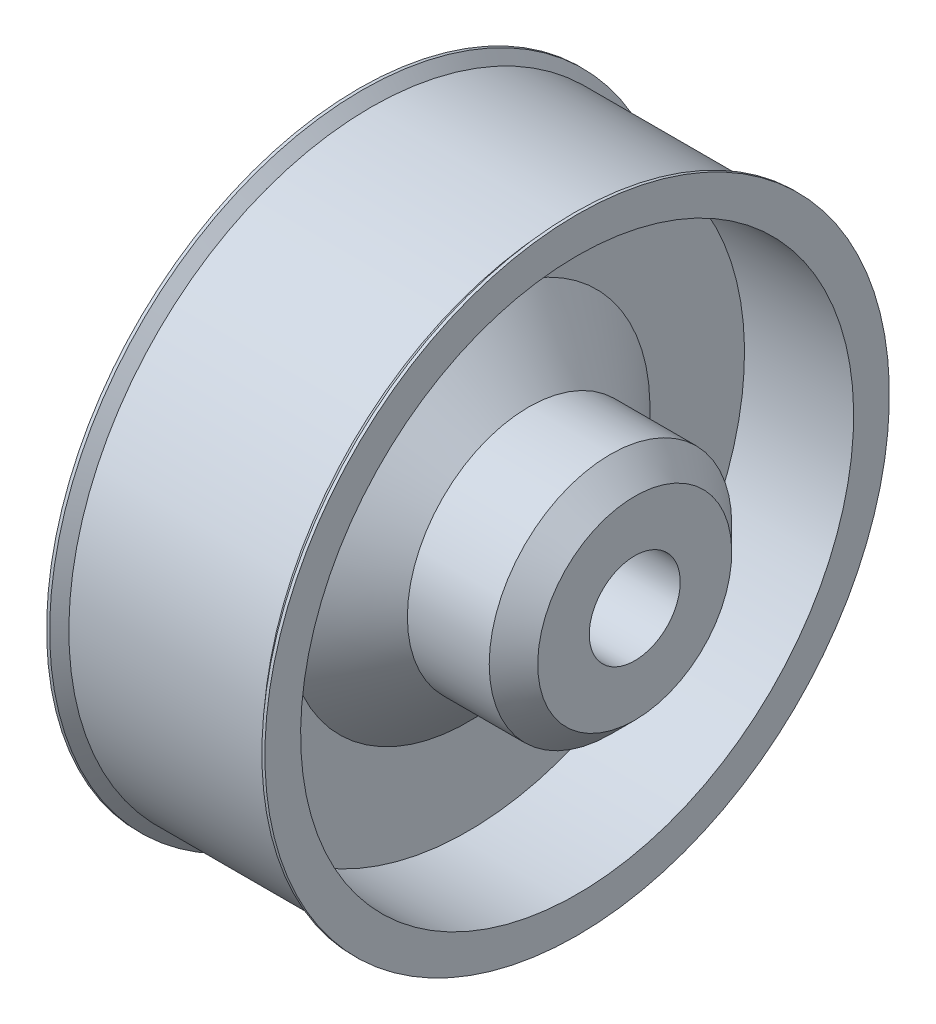
from build123d import *

# Parameters (mm, degrees)
CHAMFER1_SIZE       = 0.4
FILLET1_R           = 0.2
CHAMFER2_SIZE       = 1
BOSS_EXTRUDE1_DEPTH = 0.15
CIRPATTERN1_COUNT   = 8
BOSS_EXTRUDE2_DEPTH = 0.15
CIRPATTERN2_COUNT   = 5


with BuildPart() as part:
    # Sketch1 → Revolve1 (revolve)
    with BuildSketch(Plane.XY):
        with BuildLine():
            Line((0, 0), (0, 0.375))
            Line((0, 0.375), (1.05, 0.6))
            Line((1.05, 0.6), (1.05, 1.29376941))
            ThreePointArc((1.05, 1.29376941), (0.990535118, 1.473053702), (0.835714286, 1.581263864))
            ThreePointArc((0.835714286, 1.581263864), (0.3, 2.3), (0.835714286, 3.018736136))
            ThreePointArc((0.835714286, 3.018736136), (0.990535118, 3.126946298), (1.05, 3.30623059))
            Line((1.05, 3.30623059), (1.05, 4.231193843))
            ThreePointArc((1.05, 4.231193843), (0.953516085, 4.46412662), (0.720583307, 4.560610535))
            Line((0.720583307, 4.560610535), (0, 4.560610535))
            Line((0, 4.560610535), (0, 5.15))
            Line((0, 5.15), (0.05, 5.15))
            Line((0.05, 5.15), (0.2, 4.982919745))
            Line((0.2, 4.982919745), (3.4, 4.982919745))
            Line((3.4, 4.982919745), (3.55, 5.15))
            Line((3.55, 5.15), (3.6, 5.15))
            Line((3.6, 5.15), (3.6, 4.560610535))
            Line((3.6, 4.560610535), (1.8, 4.560610535))
            Line((1.8, 4.560610535), (1.8, 2))
            Line((1.8, 2), (4.55, 2))
            Line((4.55, 2), (4.55, 0.75))
            Line((4.55, 0.75), (1.8, 0.75))
            Line((1.8, 0.75), (1.8, 0))
            Line((1.8, 0), (0, 0))
        make_face()
    revolve(axis=Axis((1.8, 0, 0), (-1, 0, 0)))

    # Chamfer1
    chamfer1_edges = [part.edges().sort_by_distance(p)[0] for p in [
        (4.55, -2, 0),
    ]]
    chamfer(chamfer1_edges, length=CHAMFER1_SIZE)

    # Fillet1
    fillet1_edges = [part.edges().sort_by_distance(p)[0] for p in [
        (0, -4.560610535, 0),
    ]]
    fillet(fillet1_edges, radius=FILLET1_R)

    # Chamfer2
    chamfer2_edges = [part.edges().sort_by_distance(p)[0] for p in [
        (1.8, -2, 0),
    ]]
    chamfer(chamfer2_edges, length=CHAMFER2_SIZE)

    # Sketch2 → Boss-Extrude1 (add, symmetric)
    with BuildSketch(Plane.ZY.offset(-1.05)):
        Polygon((0.288675135, 3.76), (0.144337567, 4.01), (-0.144337567, 4.01), (-0.288675135, 3.76), (-0.144337567, 3.51), (0.144337567, 3.51), align=None)
    boss_extrude1 = extrude(amount=BOSS_EXTRUDE1_DEPTH, both=True)

    # CirPattern1: Boss-Extrude1 ×8 about axis
    cirpattern1_axis = Axis((0, 0, 0), (1, 0, 0))
    for i in range(1, CIRPATTERN1_COUNT):
        add(boss_extrude1.rotate(cirpattern1_axis, i * 360 / CIRPATTERN1_COUNT))

    # Sketch3 → Boss-Extrude2 (add, symmetric)
    with BuildSketch(Plane.ZY.offset(-1.05)):
        Polygon((0.288675135, 1), (0.144337567, 1.25), (-0.144337567, 1.25), (-0.288675135, 1), (-0.144337567, 0.75), (0.144337567, 0.75), align=None)
    boss_extrude2 = extrude(amount=BOSS_EXTRUDE2_DEPTH, both=True)

    # CirPattern2: Boss-Extrude2 ×5 about axis
    cirpattern2_axis = Axis((0, 0, 0), (1, 0, 0))
    for i in range(1, CIRPATTERN2_COUNT):
        add(boss_extrude2.rotate(cirpattern2_axis, i * 360 / CIRPATTERN2_COUNT))


solid = part.part
